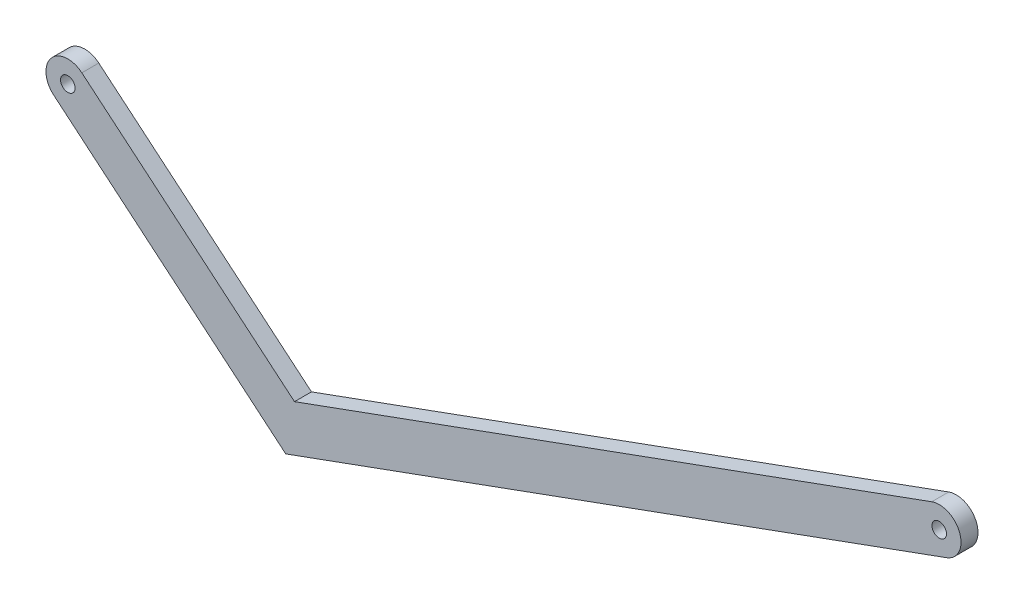
SolidWorks part; units mm, degrees
ref_plane "前视基准面" through (0, 0, 0) normal (0, 0, 1) x (1, 0, 0)
ref_plane "上视基准面" through (0, 0, 0) normal (0, 1, 0) x (1, 0, 0)
ref_plane "右视基准面" through (0, 0, 0) normal (1, 0, 0) x (0, 0, -1)
sketch "草图1" plane through (0, 0, 0) normal (0, 0, 1) x (1, 0, 0)
  line L0 (0, 0) -> (411.2456, 0) construction
  line L4 (359.4158, 20.5013) -> (91.6949, -76.9412) construction
  line L6 (362.494, 12.044) -> (89.8903, -87.1756)
  line L7 (356.3376, 28.9585) -> (93.4995, -66.7067)
  line L8 (0, 0) -> (91.6949, -76.9412) construction
  line L9 (5.7851, 6.8944) -> (93.4995, -66.7067)
  line L10 (-5.7851, -6.8944) -> (89.8903, -87.1756)
  arc A4 (362.494, 12.044) -> (356.3376, 28.9585) centre (359.4158, 20.5013) ccw
  circle A6 centre (359.4158, 20.5013) radius 3
  circle A7 centre (0, 0) radius 3
  arc A8 (5.7851, 6.8944) -> (-5.7851, -6.8944) centre (0, 0) ccw
  point P3 (201.056, -57.8509)
  point P13 (21.056, -57.8509)
  dimension "D1" = 9
  dimension "D2" = 9
  dimension "D3" = 6
  dimension "D4" = 18
  dimension "D5" = 20
  dimension "120" = 120
  dimension "D6" = 18
  dimension "D7" = 360
extrude "凸台-拉伸1" add sketch "草图1" along normal blind 7
fillet "圆角1" [suppressed] radius 8
